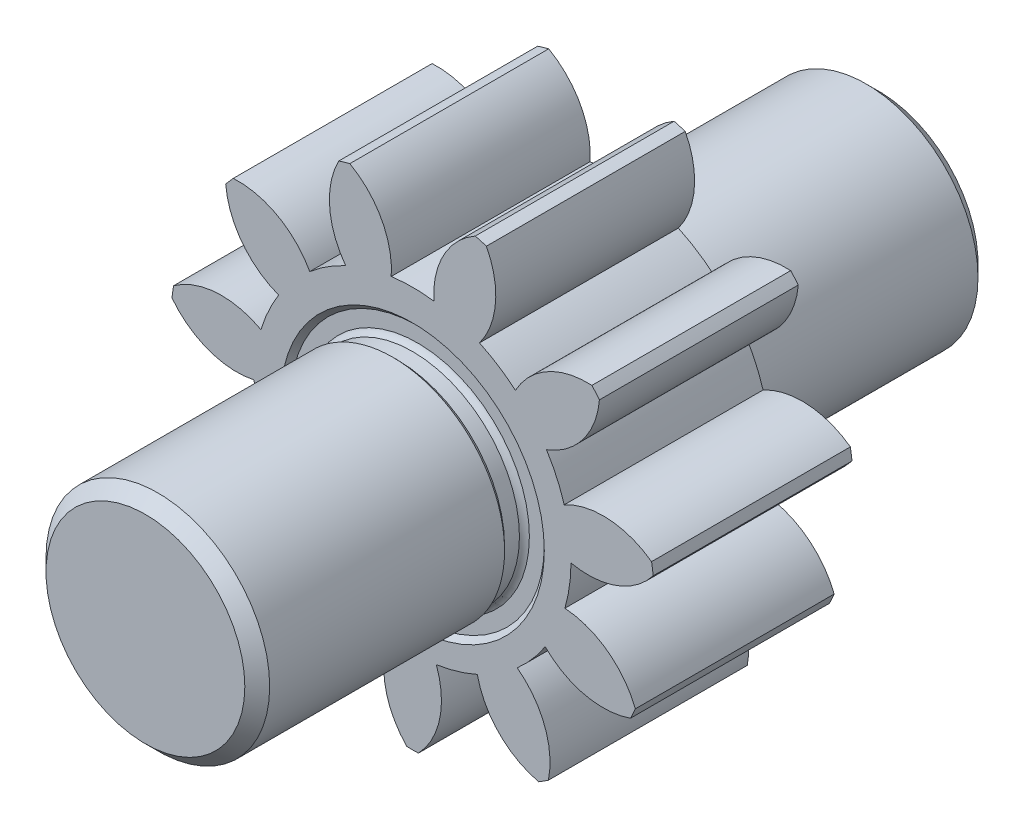
from build123d import *

# Parameters (mm, degrees)
EXTRUDE_1_DEPTH = 16
SKETCH_3_R      = 9
EXTRUDE_2_DEPTH = 21.5
CHAMFER_1_SIZE  = 1


with BuildPart() as part:
    # 草图2 → 凸台-拉伸1 (new body)
    with BuildSketch(Plane.XY):
        with BuildLine():
            ThreePointArc((-17.539719795, -8.188913461), (-13.882626521, -8.407262966), (-10.672515451, -6.641705083))
            ThreePointArc((-10.672515451, -6.641705083), (-9.635051323, -8.016686689), (-8.421711588, -9.239271212))
            ThreePointArc((-8.421711588, -9.239271212), (-10.626145075, -12.165442895), (-10.930476691, -15.816386607))
            ThreePointArc((-10.930476691, -15.816386607), (-10.54249594, -16.072311082), (-10.148525822, -16.318915917))
            ThreePointArc((-10.148525822, -16.318915917), (-6.95393453, -14.525429313), (-5.207949909, -11.304630433))
            ThreePointArc((-5.207949909, -11.304630433), (-3.591808367, -11.900443112), (-1.910102932, -12.272965675))
            ThreePointArc((-1.910102932, -12.272965675), (-2.18258254, -15.926424664), (-0.464753394, -19.162328053))
            ThreePointArc((-0.464753394, -19.162328053), (0, -19.167867192), (0.464753394, -19.162328053))
            ThreePointArc((0.464753394, -19.162328053), (2.18258254, -15.926424664), (1.910102932, -12.272965675))
            ThreePointArc((1.910102932, -12.272965675), (3.591808367, -11.900443112), (5.207949909, -11.304630433))
            ThreePointArc((5.207949909, -11.304630433), (6.95393453, -14.525429313), (10.148525822, -16.318915917))
            ThreePointArc((10.148525822, -16.318915917), (10.54249594, -16.072311082), (10.930476691, -15.816386607))
            ThreePointArc((10.930476691, -15.816386607), (10.626145075, -12.165442895), (8.421711588, -9.239271212))
            ThreePointArc((8.421711588, -9.239271212), (9.635051323, -8.016686689), (10.672515451, -6.641705083))
            ThreePointArc((10.672515451, -6.641705083), (13.882626521, -8.407262966), (17.539719795, -8.188913461))
            ThreePointArc((17.539719795, -8.188913461), (17.737823909, -7.768459945), (17.925850869, -7.343404347))
            ThreePointArc((17.925850869, -7.343404347), (15.69598163, -4.436569144), (12.25948632, -3.166723601))
            ThreePointArc((12.25948632, -3.166723601), (12.619233563, -1.482239065), (12.748632746, 0.235364522))
            ThreePointArc((12.748632746, 0.235364522), (16.403682682, 0.485599789), (19.362176663, 2.646460979))
            ThreePointArc((19.362176663, 2.646460979), (19.301518117, 3.107272155), (19.229894055, 3.566506728))
            ThreePointArc((19.229894055, 3.566506728), (15.782454919, 4.806333783), (12.204960767, 4.016686199))
            ThreePointArc((12.204960767, 4.016686199), (11.596898309, 5.628258809), (10.777149222, 7.143157375))
            ThreePointArc((10.777149222, 7.143157375), (13.716685494, 9.329737862), (15.037279247, 12.747052577))
            ThreePointArc((15.037279247, 12.747052577), (14.7371167, 13.10191712), (14.42858175, 13.449526936))
            ThreePointArc((14.42858175, 13.449526936), (10.858110285, 12.628709513), (8.275446406, 10.030276331))
            ThreePointArc((8.275446406, 10.030276331), (6.892629782, 11.057274099), (5.383996967, 11.888498053))
            ThreePointArc((5.383996967, 11.888498053), (6.674737579, 15.317199905), (5.938151919, 18.905994868))
            ThreePointArc((5.938151919, 18.905994868), (5.493784858, 19.042245794), (5.046296687, 19.167867192))
            ThreePointArc((5.046296687, 19.167867192), (2.486392356, 16.547009024), (1.718536283, 12.964774418))
            ThreePointArc((1.718536283, 12.964774418), (0, 13.081132808), (-1.718536283, 12.964774418))
            ThreePointArc((-1.718536283, 12.964774418), (-2.486392356, 16.547009024), (-5.046296687, 19.167867192))
            ThreePointArc((-5.046296687, 19.167867192), (-5.493784858, 19.042245794), (-5.938151919, 18.905994868))
            ThreePointArc((-5.938151919, 18.905994868), (-6.674737579, 15.317199905), (-5.383996967, 11.888498053))
            ThreePointArc((-5.383996967, 11.888498053), (-6.892629782, 11.057274099), (-8.275446406, 10.030276331))
            ThreePointArc((-8.275446406, 10.030276331), (-10.858110285, 12.628709513), (-14.42858175, 13.449526936))
            ThreePointArc((-14.42858175, 13.449526936), (-14.7371167, 13.10191712), (-15.037279247, 12.747052577))
            ThreePointArc((-15.037279247, 12.747052577), (-13.716685494, 9.329737862), (-10.777149222, 7.143157375))
            ThreePointArc((-10.777149222, 7.143157375), (-11.596898309, 5.628258809), (-12.204960767, 4.016686199))
            ThreePointArc((-12.204960767, 4.016686199), (-15.782454919, 4.806333783), (-19.229894055, 3.566506728))
            ThreePointArc((-19.229894055, 3.566506728), (-19.301518117, 3.107272155), (-19.362176663, 2.646460979))
            ThreePointArc((-19.362176663, 2.646460979), (-16.403682682, 0.485599789), (-12.748632746, 0.235364522))
            ThreePointArc((-12.748632746, 0.235364522), (-12.619233563, -1.482239065), (-12.25948632, -3.166723601))
            ThreePointArc((-12.25948632, -3.166723601), (-15.69598163, -4.436569144), (-17.925850869, -7.343404347))
            ThreePointArc((-17.925850869, -7.343404347), (-17.737823909, -7.768459945), (-17.539719795, -8.188913461))
        make_face()
    extrude(amount=EXTRUDE_1_DEPTH)

    # 草图3 → 凸台-拉伸2 (add)
    with BuildSketch(Plane.XY.offset(16)):
        Circle(SKETCH_3_R)
    extrude_2 = extrude(amount=EXTRUDE_2_DEPTH)

    # 草图4 → 切除-旋转1 (revolve, cut)
    with BuildSketch(Plane(origin=(0, 0, 0), x_dir=(0, 0, -1), z_dir=(1, 0, 0)), mode=Mode.PRIVATE) as cut_revolve_1_sk:
        with BuildLine():
            Line((-17.6, 8.999602816), (-17.2, 8.599602816))
            Line((-17.2, 8.599602816), (-16, 8.599602816))
            ThreePointArc((-16, 8.599602816), (-15.763464837, 8.763067654), (-15.6, 8.999602816))
            Line((-15.6, 8.999602816), (-15.6, 10.199602816))
            Line((-15.6, 10.199602816), (-16, 10.599602816))
            Line((-16, 10.599602816), (-17.6, 10.599602816))
            Line((-17.6, 10.599602816), (-17.6, 8.999602816))
        make_face()
    cut_revolve_1 = revolve(cut_revolve_1_sk.sketch.rotate(Axis((0, 0, 37.5), (0, 0, -1)), 90), axis=Axis((0, 0, 37.5), (0, 0, -1)), mode=Mode.SUBTRACT)

    # 镜向1: 凸台-拉伸2, 切除-旋转1 across plane
    add(extrude_2.mirror(Plane.XY.offset(8)))
    add(cut_revolve_1.mirror(Plane.XY.offset(8)), mode=Mode.SUBTRACT)

    # 倒角1
    chamfer_1_edges = [part.edges().sort_by_distance(p)[0] for p in [
        (-9, 0, 37.5),
        (-9, 0, -21.5),
    ]]
    chamfer(chamfer_1_edges, length=CHAMFER_1_SIZE)


solid = part.part
